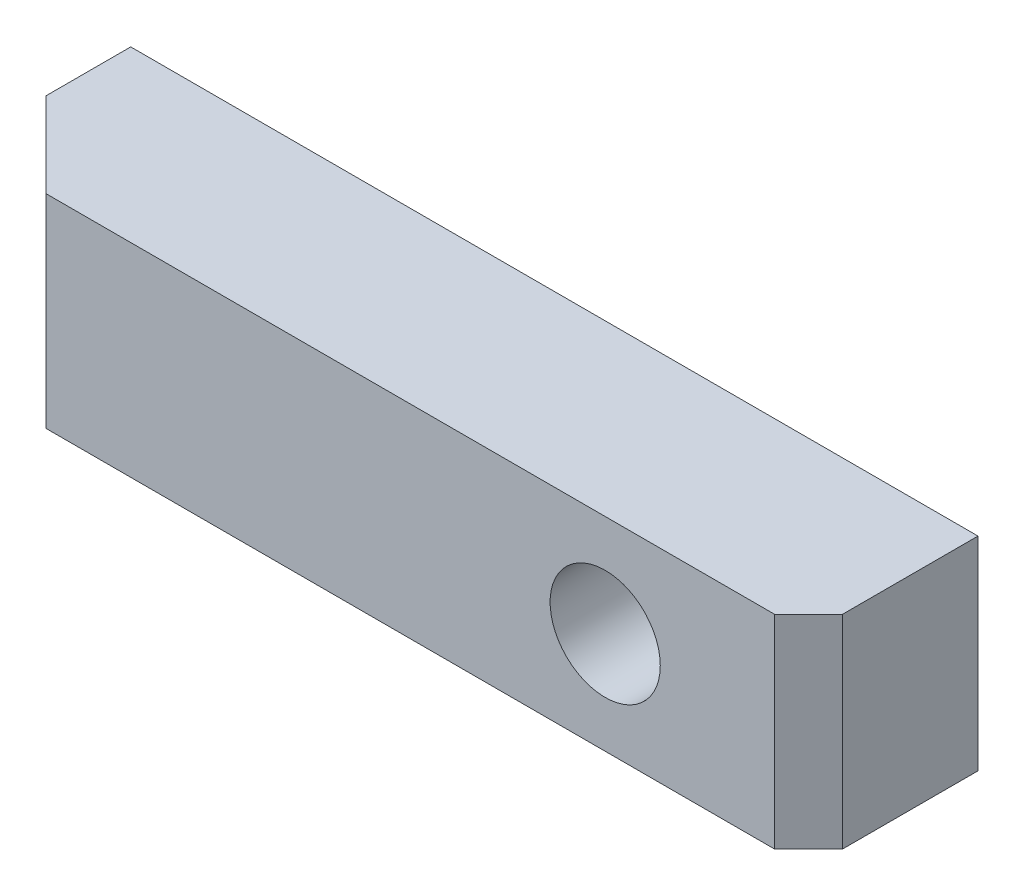
from build123d import *

# Parameters (mm, degrees)
BOSS_EXTRUDE1_DEPTH        = 12
F_6_5_6_5_DIAMETER_HOLE1_D = 6.5
CHAMFER1_SIZE              = 2


with BuildPart() as part:
    # Sketch1 → Boss-Extrude1 (new body)
    with BuildSketch(Plane(origin=(0, 6, 0), x_dir=(1, 0, 0), z_dir=(0, 1, 0))):
        Polygon((-20, -5), (25, -5), (25, 5), (-25, 5), (-25, 0), align=None)
    extrude(amount=-BOSS_EXTRUDE1_DEPTH)

    # Ø6.5 (6.5) Diameter Hole1 (through all)
    with Locations(Plane.XY.offset(5)):
        with Locations((13, 0)):
            Hole(F_6_5_6_5_DIAMETER_HOLE1_D / 2)

    # Chamfer1
    chamfer1_edges = [part.edges().sort_by_distance(p)[0] for p in [
        (25, 0, 5),
    ]]
    chamfer(chamfer1_edges, length=CHAMFER1_SIZE)


solid = part.part
